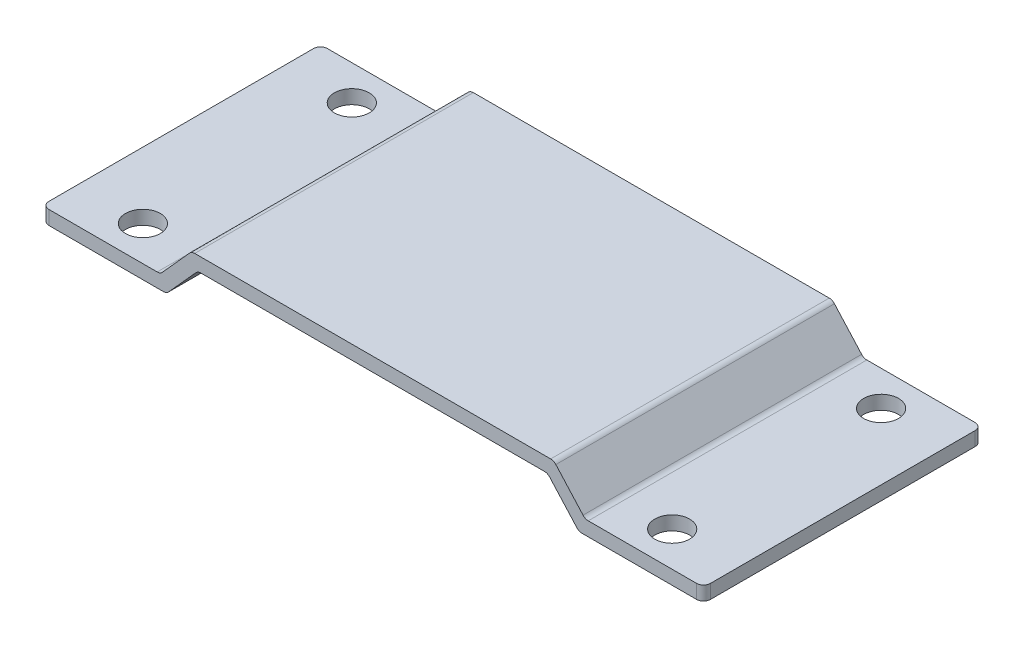
from build123d import *

# Parameters (mm, degrees)
BOSS_EXTRUDE1_DEPTH      = 20
BOSS_EXTRUDE1_DEPTH_BACK = 20
SKETCH2_R                = 2.5
CUT_EXTRUDE1_DEPTH       = 20
FILLET1_R                = 1


with BuildPart() as part:
    # Sketch1 → Boss-Extrude1 (new, two sides: drawn at the far end of the back side and taken through both)
    with BuildSketch(Plane.XY.offset(-BOSS_EXTRUDE1_DEPTH_BACK)):
        with BuildLine():
            Line((-47.5, 0), (-30.945362405, 0))
            ThreePointArc((-30.945362405, 0), (-30.53852382, 0.086499937), (-30.202068258, 0.331035268))
            Line((-30.202068258, 0.331035268), (-26.297931742, 4.668964732))
            ThreePointArc((-26.297931742, 4.668964732), (-25.96147618, 4.913500063), (-25.554637595, 5))
            Line((-25.554637595, 5), (25.554637595, 5))
            ThreePointArc((25.554637595, 5), (25.96147618, 4.913500063), (26.297931742, 4.668964732))
            Line((26.297931742, 4.668964732), (30.202068258, 0.331035268))
            ThreePointArc((30.202068258, 0.331035268), (30.53852382, 0.086499937), (30.945362405, 0))
            Line((30.945362405, 0), (47.5, 0))
            Line((47.5, 0), (47.5, -2))
            Line((47.5, -2), (30.054637595, -2))
            ThreePointArc((30.054637595, -2), (29.64779901, -1.913500063), (29.311343449, -1.668964732))
            Line((29.311343449, -1.668964732), (25.407206932, 2.668964732))
            ThreePointArc((25.407206932, 2.668964732), (25.070751371, 2.913500063), (24.663912786, 3))
            Line((24.663912786, 3), (-24.663912786, 3))
            ThreePointArc((-24.663912786, 3), (-25.070751371, 2.913500063), (-25.407206932, 2.668964732))
            Line((-25.407206932, 2.668964732), (-29.311343449, -1.668964732))
            ThreePointArc((-29.311343449, -1.668964732), (-29.64779901, -1.913500063), (-30.054637595, -2))
            Line((-30.054637595, -2), (-47.5, -2))
            Line((-47.5, -2), (-47.5, 0))
        make_face()
    extrude(amount=BOSS_EXTRUDE1_DEPTH + BOSS_EXTRUDE1_DEPTH_BACK)

    # Sketch2 → Cut-Extrude1 (cut)
    with BuildSketch(Plane(origin=(0, 0, 0), x_dir=(1, 0, 0), z_dir=(0, 1, 0))):
        with Locations(Location((-38, 15, 0), (0, 0, 180))):
            Circle(SKETCH2_R)
        with Locations(Location((38, 15, 0), (0, 0, 90))):
            Circle(SKETCH2_R)
        with Locations(Location((38, -15, 0), (0, 0, 180))):
            Circle(SKETCH2_R)
        with Locations(Location((-38, -15, 0), (0, 0, 90))):
            Circle(SKETCH2_R)
    extrude(amount=-CUT_EXTRUDE1_DEPTH, mode=Mode.SUBTRACT)

    # Fillet1
    fillet1_edges = [part.edges().sort_by_distance(p)[0] for p in [
        (47.5, -1, -20),
        (-47.5, -1, -20),
        (-47.5, -1, 20),
        (47.5, -1, 20),
    ]]
    fillet(fillet1_edges, radius=FILLET1_R)


solid = part.part
